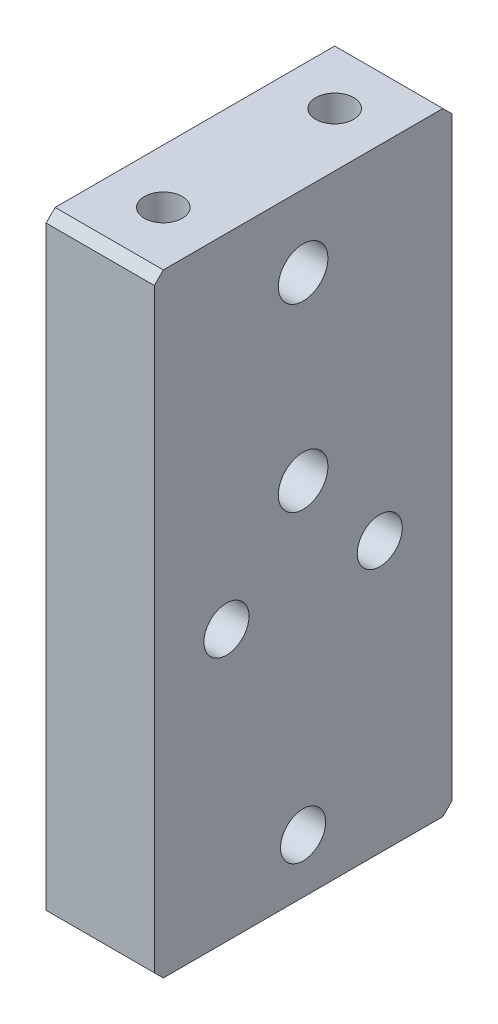
from build123d import *

# Parameters (mm, degrees)
SKETCH_1_W                  = 12
SKETCH_1_H                  = 68
EXTRUDE_1_DEPTH             = 33
HOLE_WIZARD_M6_1_D          = 5
HOLE_WIZARD_M6_1_DEPTH      = 15
HOLE_WIZARD_M6_1_TIP        = 1.502151548
HOLE_WIZARD_M5_1_D          = 4.2
HOLE_WIZARD_M5_1_DEPTH      = 11
HOLE_WIZARD_M5_1_TIP        = 1.2618073
HOLE_WIZARD_C_0_D           = 5.5
HOLE_WIZARD_C_0_CBORE_D     = 10
HOLE_WIZARD_C_0_CBORE_DEPTH = 5.5
CHAMFER_1_SIZE              = 1


with BuildPart() as part:
    # 草图1 → 凸台-拉伸1 (new body)
    with BuildSketch(Plane.XY):
        with Locations((-70.482202682, -45.607833778)):
            Rectangle(SKETCH_1_W, SKETCH_1_H)
    extrude(amount=-EXTRUDE_1_DEPTH)

    # M6 螺纹孔1
    with Locations(Plane.ZY.offset(76.482202682)):
        with Locations((-16.5, -73.607833778), (-8, -49.607833778), (-25, -49.607833778)):
            Hole(HOLE_WIZARD_M6_1_D / 2, depth=HOLE_WIZARD_M6_1_DEPTH)
            with Locations((0, 0, -(HOLE_WIZARD_M6_1_DEPTH + HOLE_WIZARD_M6_1_TIP / 2))):  # 118° drill point
                Cone(0, HOLE_WIZARD_M6_1_D / 2, HOLE_WIZARD_M6_1_TIP, mode=Mode.SUBTRACT)

    # M5 螺纹孔1
    with Locations(Plane(origin=(0, -11.607833778, 0), x_dir=(1, 0, 0), z_dir=(0, 1, 0))):
        with Locations((-70.482202682, 26), (-70.482202682, 7)):
            Hole(HOLE_WIZARD_M5_1_D / 2, depth=HOLE_WIZARD_M5_1_DEPTH)
            with Locations((0, 0, -(HOLE_WIZARD_M5_1_DEPTH + HOLE_WIZARD_M5_1_TIP / 2))):  # 118° drill point
                Cone(0, HOLE_WIZARD_M5_1_D / 2, HOLE_WIZARD_M5_1_TIP, mode=Mode.SUBTRACT)

    # 打孔尺寸根据六角头螺栓 C 级的类型0 (through all)
    with Locations(Plane.ZY.offset(76.482202682)):
        with Locations((-16.5, -19.604255019), (-16.5, -39.607833778)):
            CounterBoreHole(HOLE_WIZARD_C_0_D / 2, HOLE_WIZARD_C_0_CBORE_D / 2, HOLE_WIZARD_C_0_CBORE_DEPTH)

    # 倒角1
    chamfer_1_edges = [part.edges().sort_by_distance(p)[0] for p in [
        (-70.482202682, -11.607833778, -33),
        (-70.482202682, -11.607833778, 0),
        (-70.482202682, -79.607833778, 0),
        (-70.482202682, -79.607833778, -33),
    ]]
    chamfer(chamfer_1_edges, length=CHAMFER_1_SIZE)


solid = part.part
